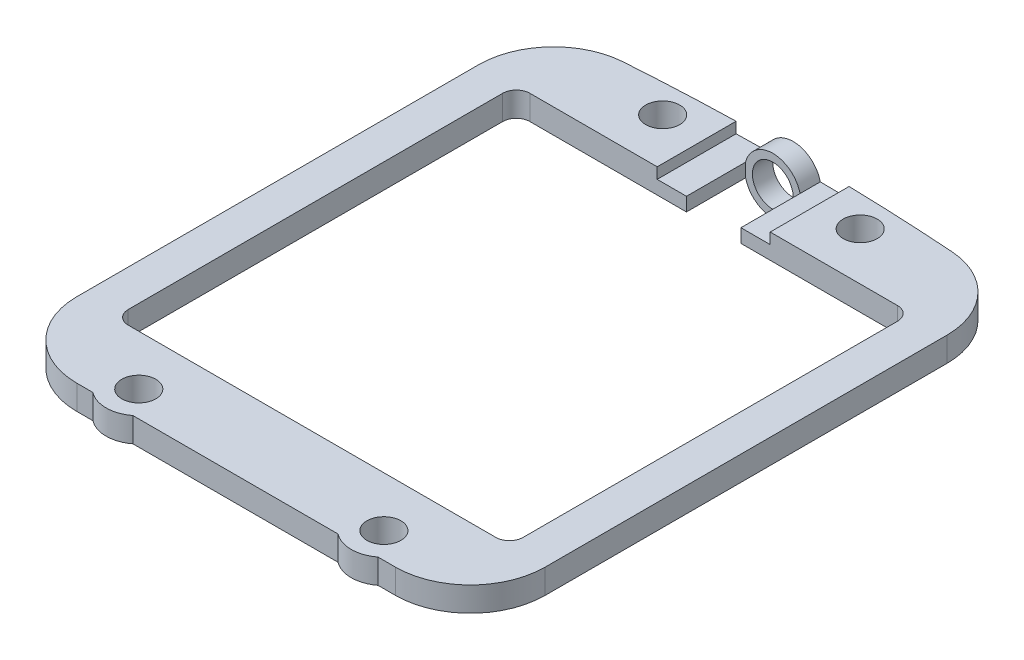
SolidWorks part; units mm, degrees
material "ABS"
ref_plane "Front Plane" through (0, 0, 0) normal (0, 0, 1) x (1, 0, 0)
ref_plane "Top Plane" through (0, 0, 0) normal (0, 1, 0) x (1, 0, 0)
ref_plane "Right Plane" through (0, 0, 0) normal (1, 0, 0) x (0, 0, -1)
sketch "Sketch 1" plane through (0, 0, 0) normal (0, 1, 0) x (1, 0, 0)
  line L0 (-17.2, -14.827) -> (-17.2, 14.6862)
  line L1 (-13.5, -14.75) -> (13.5, -14.75)
  line L2 (-14.5, -13.75) -> (-14.5, 13.75)
  line L3 (-13.5, 14.75) -> (13.5, 14.75)
  line L4 (14.5, -13.75) -> (14.5, 13.75)
  line L5 (-14.5, -14.75) -> (14.5, 14.75) construction
  line L6 (-14.5, 14.75) -> (14.5, -14.75) construction
  line L7 (17.2, -14.827) -> (17.2, 14.6862)
  line L8 (-7.5837, -20.327) -> (7.4874, -20.327)
  line L9 (10.42, -20.327) -> (11.7, -20.327)
  line L10 (17.2, -14.75) -> (17.2, 14.75) construction
  line L11 (-17.2, -14.75) -> (-17.2, 14.75) construction
  line L13 (-14.5, -14.75) -> (-14.5, 14.75) construction
  line L14 (14.5, -14.75) -> (14.5, 14.75) construction
  line L15 (-11.7, -20.327) -> (-10.5163, -20.327)
  arc A0 (-12.0819, 20.173) -> (12.0819, 20.173) centre (0, -153.3944) cw
  arc A1 (17.2, 14.6862) -> (12.0819, 20.173) centre (11.7, 14.6862) ccw
  arc A2 (-12.0819, 20.173) -> (-17.2, 14.6862) centre (-11.7, 14.6862) ccw
  arc A3 (11.7, -20.327) -> (17.2, -14.827) centre (11.7, -14.827) ccw
  arc A4 (-11.7, -20.327) -> (-17.2, -14.827) centre (-11.7, -14.827) cw
  arc A5 (-13.5, -14.75) -> (-14.5, -13.75) centre (-13.5, -13.75) cw
  arc A6 (13.5, -14.75) -> (14.5, -13.75) centre (13.5, -13.75) ccw
  arc A7 (14.5, 13.75) -> (13.5, 14.75) centre (13.5, 13.75) ccw
  arc A8 (-14.5, 13.75) -> (-13.5, 14.75) centre (-13.5, 13.75) cw
  arc A10 (-10.5163, -20.327) -> (-7.5837, -20.327) centre (-9.05, -18.427) ccw
  arc A12 (7.4874, -20.327) -> (10.42, -20.327) centre (8.9537, -18.427) ccw
  point P0 (0, 0)
  dimension "D6" = 5.5
  dimension "D7" = 1
  dimension "D8" = 4.8
  dimension "D9" = 0.5
  dimension "D5" = 4.8
  dimension "D1" = 29
  dimension "D2" = 29.5
  dimension "D10" = 40.92
  dimension "D11" = 40.5
  dimension "D3" = 2.7
  dimension "D4" = 2.7
extrude "Boss-Extrude 1" add sketch "Sketch 1" along normal mid plane 1.8
sketch "Sketch 2" plane through (0, 0, 0) normal (0, 1, 0) x (1, 0, 0)
  circle A0 centre (-9.05, -18.427) radius 1.25
  circle A1 centre (8.9537, -18.427) radius 1.25
  circle A2 centre (-7.2531, 18.2569) radius 1.25
  circle A3 centre (7.2531, 18.2569) radius 1.25
  arc A4 (-6.5082, 18.2833) -> (-7.998, 18.2276) centre (0, -175.4941) ccw construction
  arc A5 (7.998, 18.2276) -> (6.5082, 18.2833) centre (0, -175.4941) ccw construction
  dimension "D1" = 2.5
  dimension "D2" = 2.5
  dimension "D3" = 2.5
  dimension "D4" = 2.5
extrude "Cut-Extrude 1" cut sketch "Sketch 2" against normal through all and the other way through all
sketch "Sketch 3" plane through (0, 0.9, 0) normal (0, 1, 0) x (1, 0, 0)
  line L0 (2, 14.75) -> (-2, 14.75)
  line L1 (2, 14.75) -> (2, 19.093)
  line L2 (-2, 14.75) -> (-2, 19.093)
  line L3 (2, 19.093) -> (-2, 19.093)
  line L4 (13.5, 14.75) -> (-13.5, 14.75) construction
  arc A1 (12.0819, 20.173) -> (-12.0819, 20.173) centre (0, -153.3944) ccw construction
  point P4 (0, 14.75)
  dimension "D1" = 4
  dimension "D2" = 1.5
extrude "Cut-Extrude 2" cut sketch "Sketch 3" against normal blind 1.8
sketch "Sketch 4" plane through (0, 0.9, 0) normal (0, 1, 0) x (1, 0, 0)
  line L2 (4.15, 14.75) -> (-4.15, 14.75)
  line L3 (-4.15, 20.9253) -> (-4.15, 14.75)
  line L4 (0, 0) -> (0, 26.4288) construction
  line L5 (4.15, 20.9253) -> (4.15, 14.75)
  line L7 (-4.15, 20.9253) -> (4.15, 20.9253)
  dimension "D1" = 8.3
extrude "Cut-Extrude3" cut sketch "Sketch 4" against normal blind 0.8
sketch "Sketch 10" plane through (0, 0, -19.093) normal (0, 0, 1) x (1, 0, 0)
  circle A0 centre (0, -0.4) radius 2.0616
  circle A1 centre (0, -0.4) radius 1.5
  dimension "D1" = 3
  dimension "D2" = 4.1231
extrude "Boss-Extrude 2" add sketch "Sketch 10" against normal up to surface (1.4878 mm away)
sketch "Sketch 11" plane through (0, 0, -19.093) normal (0, 0, 1) x (1, 0, 0)
  circle A0 centre (0, -0.4) radius 1.5
  arc A1 (-1.4142, -0.9) -> (1.4142, -0.9) centre (0, -0.4) ccw construction
extrude "Cut-Extrude 7" cut sketch "Sketch 11" against normal blind 10
